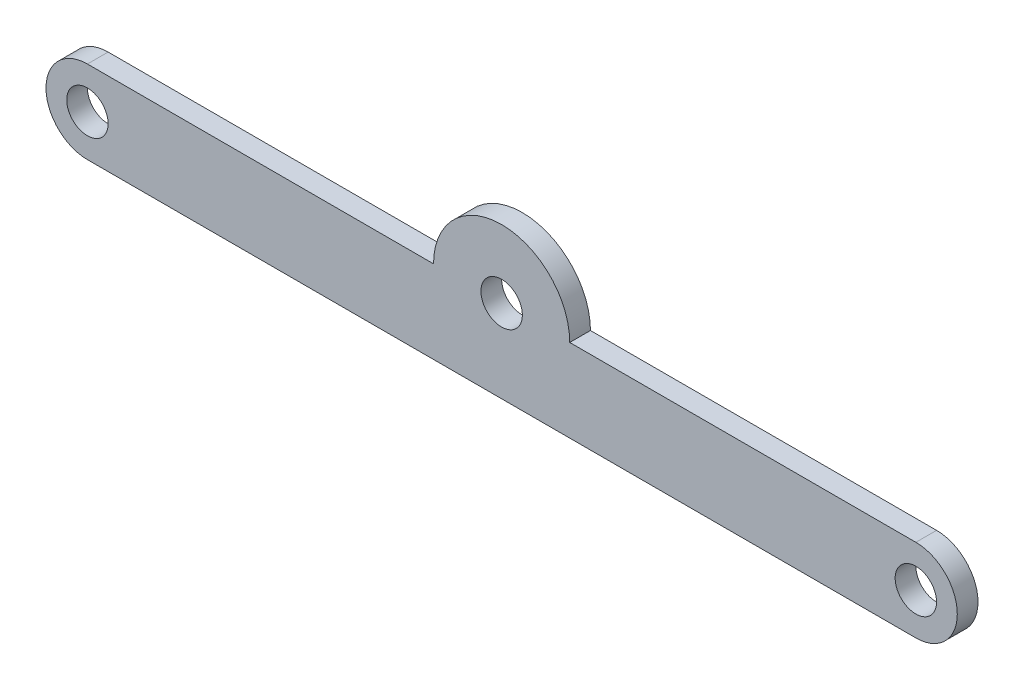
from build123d import *

# Parameters (mm, degrees)
BOSS_EXTRUDE1_DEPTH = 10
SKETCH2_R           = 10
CUT_EXTRUDE1_DEPTH  = 222.133443875
SKETCH4_R           = 32.878916004
BOSS_EXTRUDE2_DEPTH = 10
SKETCH5_R           = 10
CUT_EXTRUDE3_DEPTH  = 227.48659951


with BuildPart() as part:
    # Sketch1 → Boss-Extrude1 (new body)
    with BuildSketch(Plane.XY):
        with BuildLine():
            Line((-200, 20), (200, 20))
            ThreePointArc((200, 20), (220, 0), (200, -20))
            Line((200, -20), (-200, -20))
            ThreePointArc((-200, -20), (-220, 0), (-200, 20))
        make_face()
    extrude(amount=BOSS_EXTRUDE1_DEPTH)

    # Sketch2 → Cut-Extrude1 (cut, through all)
    with BuildSketch(Plane.XY.offset(10)):
        with Locations((-200, 0)):
            Circle(SKETCH2_R)
        with Locations((200, 0)):
            Circle(SKETCH2_R)
    extrude(amount=-CUT_EXTRUDE1_DEPTH, mode=Mode.SUBTRACT)

    # Sketch4 → Boss-Extrude2 (add)
    with BuildSketch(Plane.XY.offset(10)):
        with Locations((0, 20)):
            Circle(SKETCH4_R)
    extrude(amount=-BOSS_EXTRUDE2_DEPTH)

    # Sketch5 → Cut-Extrude3 (cut, through all)
    with BuildSketch(Plane.XY.offset(10)):
        with Locations((0, 20)):
            Circle(SKETCH5_R)
    extrude(amount=-CUT_EXTRUDE3_DEPTH, mode=Mode.SUBTRACT)


solid = part.part
